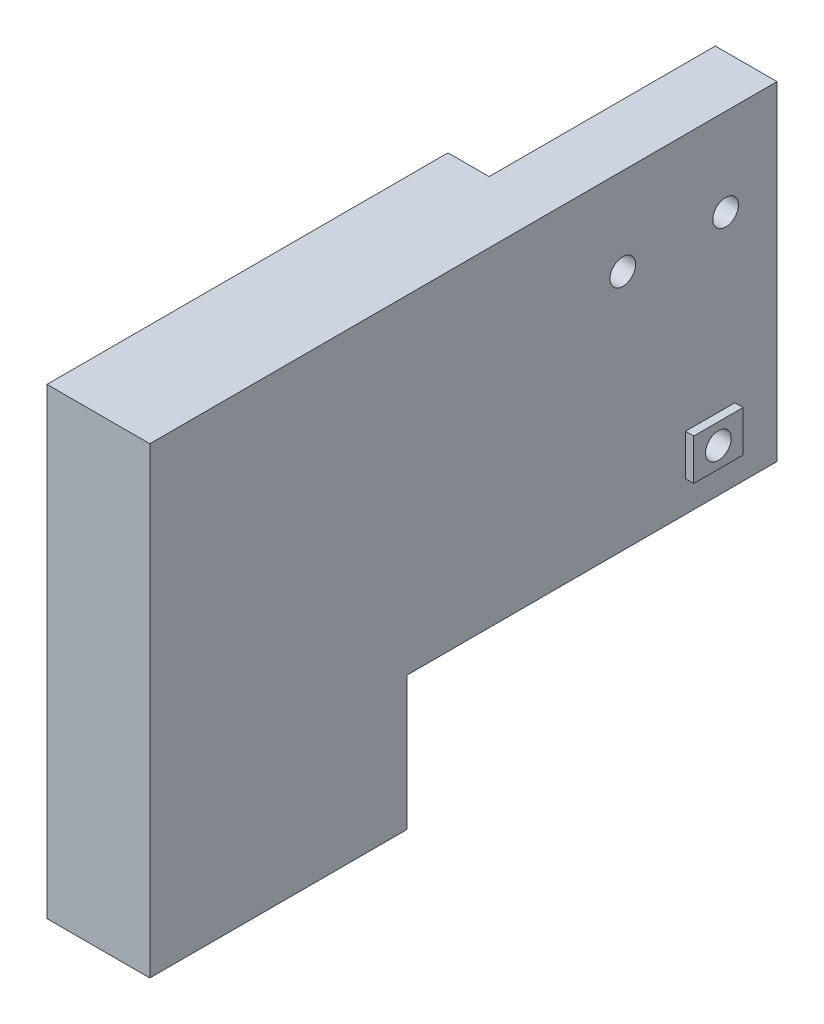
from build123d import *

# Parameters (mm, degrees)
EXTRUDE_THIN1_DEPTH   = 25
SKETCH2_W             = 36
SKETCH2_H             = 32
BOSS_EXTRUDE1_DEPTH   = 10
SKETCH5_W             = 4
SKETCH5_H             = 22
CUT_EXTRUDE1_DEPTH    = 68.424031324
SKETCH6_W             = 55.512258346
SKETCH6_H             = 44.910131752
CUT_EXTRUDE2_DEPTH    = 10
M5_TAPPED_HOLE1_D     = 4.2
M5_TAPPED_HOLE1_DEPTH = 12.4
M5_TAPPED_HOLE1_TIP   = 1.2618073
M3_TAPPED_HOLE1_D     = 2.5
SKETCH11_W            = 4.8
SKETCH11_H            = 4
BOSS_EXTRUDE2_DEPTH   = 0.8
M3_TAPPED_HOLE2_D     = 2.5


with BuildPart() as part:
    # Sketch1 → Extrude-Thin1 (new body)
    with BuildSketch(Plane.XY):
        Polygon((-15, 0), (0, 0), (0, 45), (10, 45), (10, -10), (-15, -10), align=None)
    extrude(amount=EXTRUDE_THIN1_DEPTH)

    # Sketch2 → Boss-Extrude1 (add)
    with BuildSketch(Plane.ZY):
        with Locations((-18, 29)):
            Rectangle(SKETCH2_W, SKETCH2_H)
    extrude(amount=-BOSS_EXTRUDE1_DEPTH)

    # Sketch5 → Cut-Extrude1 (cut, through all)
    with BuildSketch(Plane(origin=(0, 45, 0), x_dir=(1, 0, 0), z_dir=(0, 1, 0))):
        with Locations((2, 25)):
            Rectangle(SKETCH5_W, SKETCH5_H)
    extrude(amount=-CUT_EXTRUDE1_DEPTH, mode=Mode.SUBTRACT)

    # Sketch6 → Cut-Extrude2 (cut)
    with BuildSketch(Plane.XZ.offset(10)):
        with Locations((-2.5, 9.73543964)):
            Rectangle(SKETCH6_W, SKETCH6_H)
    extrude(amount=-CUT_EXTRUDE2_DEPTH, mode=Mode.SUBTRACT)

    # M5 Tapped Hole1
    with Locations(Plane(origin=(0, 0, 0), x_dir=(-1, 0, 0), z_dir=(0, -1, 0))):
        with Locations((-5, -5.5), (-5, -19.5)):
            Hole(M5_TAPPED_HOLE1_D / 2, depth=M5_TAPPED_HOLE1_DEPTH)
            with Locations((0, 0, -(M5_TAPPED_HOLE1_DEPTH + M5_TAPPED_HOLE1_TIP / 2))):  # 118° drill point
                Cone(0, M5_TAPPED_HOLE1_D / 2, M5_TAPPED_HOLE1_TIP, mode=Mode.SUBTRACT)

    # M3 Tapped Hole1 (through all)
    with Locations(Plane.ZY.offset(-4)):
        with Locations((-31, 36.5), (-21, 36.5)):
            Hole(M3_TAPPED_HOLE1_D / 2)

    # Sketch11 → Boss-Extrude2 (add)
    with BuildSketch(Plane(origin=(10, 0, 0), x_dir=(0, 0, -1), z_dir=(1, 0, 0))):
        with Locations((29.5, 18)):
            Rectangle(SKETCH11_W, SKETCH11_H)
    extrude(amount=BOSS_EXTRUDE2_DEPTH)

    # M3 Tapped Hole2 (through all)
    with Locations(Plane.ZY):
        with Locations((-29.5, 18)):
            Hole(M3_TAPPED_HOLE2_D / 2)


solid = part.part
